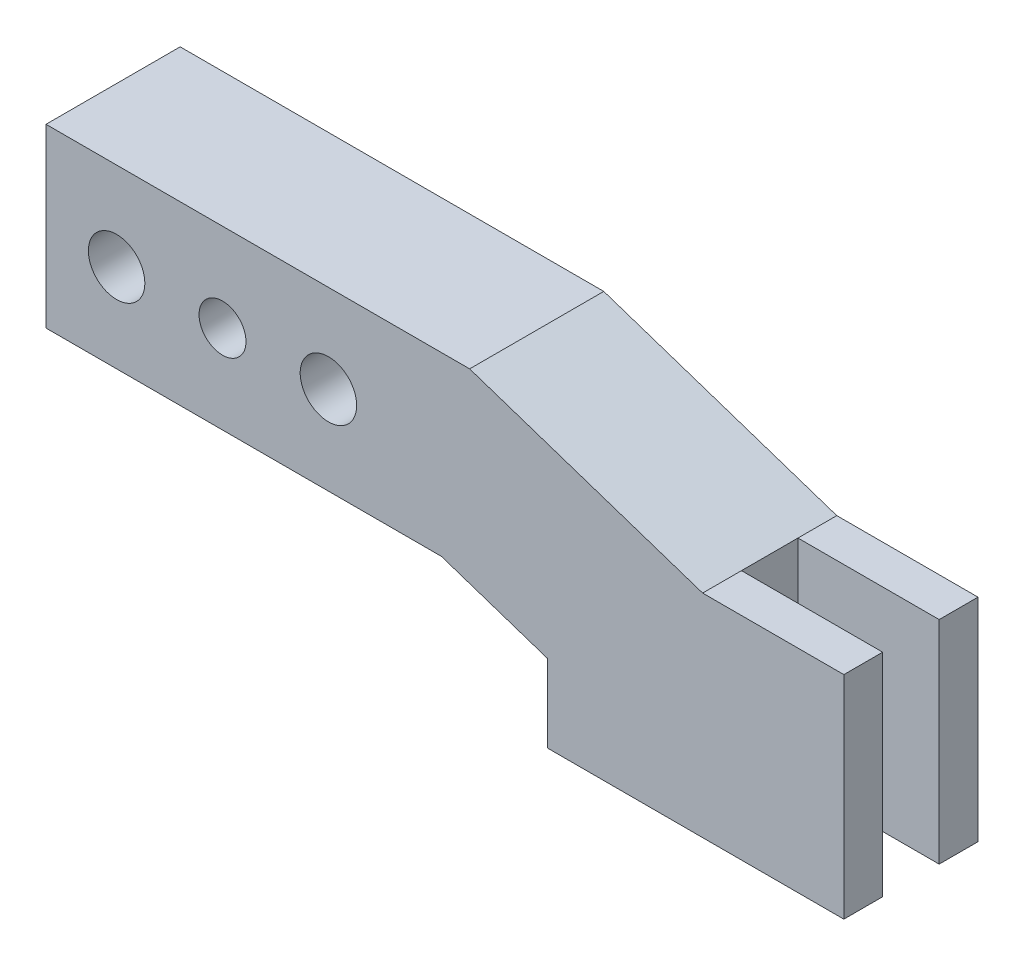
from build123d import *

# Parameters (mm, degrees)
SKETCH1_R           = 4
SKETCH1_R_2         = 3.3235
BOSS_EXTRUDE1_DEPTH = 19
CUT_EXTRUDE1_REACH  = 120.448
SKETCH2_W           = 20
SKETCH2_H           = 8
SKETCH3_R           = 2.4585
CUT_EXTRUDE2_DEPTH  = 15


with BuildPart() as part:
    # Sketch1 → Boss-Extrude1 (new body)
    with BuildSketch(Plane.XY):
        Polygon((0, 0), (56, 0), (71, -5), (71, -16), (113, -16), (113, 14), (93, 14), (60, 25), (0, 25), align=None)
        with Locations((10, 12.5)):
            Circle(SKETCH1_R, mode=Mode.SUBTRACT)
        with Locations((25, 12.5)):
            Circle(SKETCH1_R_2, mode=Mode.SUBTRACT)
        with Locations((40, 12.5)):
            Circle(SKETCH1_R, mode=Mode.SUBTRACT)
    extrude(amount=BOSS_EXTRUDE1_DEPTH)

    # Sketch2 → Cut-Extrude1 (cut, up to next)
    with BuildSketch(Plane(origin=(0, 14, 0), x_dir=(1, 0, 0), z_dir=(0, 1, 0)), mode=Mode.PRIVATE) as cut_extrude1_sk1:
        with Locations((103, -9.5)):
            Rectangle(SKETCH2_W, SKETCH2_H)
    cut_extrude1_tool1 = extrude(cut_extrude1_sk1.sketch, amount=-CUT_EXTRUDE1_REACH, mode=Mode.PRIVATE) & part.part
    add(cut_extrude1_tool1.solids().sort_by_distance((103, 14, 9.5))[0], mode=Mode.SUBTRACT)

    # Sketch3 → Cut-Extrude2 (cut)
    with BuildSketch(Plane(origin=(0, -16, 0), x_dir=(-1, 0, 0), z_dir=(0, -1, 0))):
        with Locations(Location((-79, -9.5, 0), (0, 0, 180))):
            Circle(SKETCH3_R)
    extrude(amount=-CUT_EXTRUDE2_DEPTH, mode=Mode.SUBTRACT)


solid = part.part
